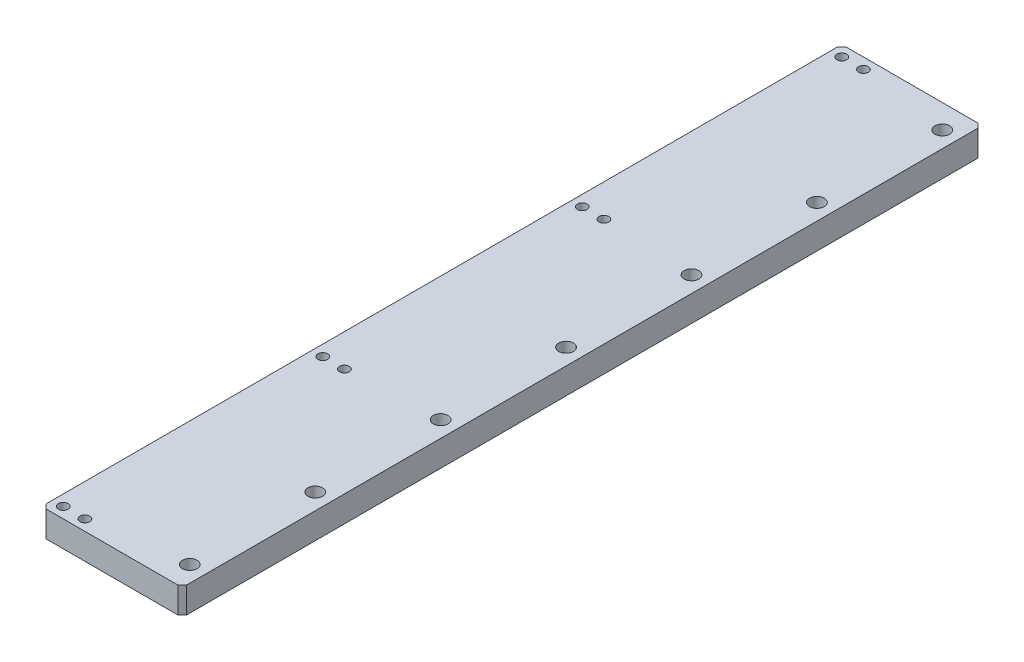
from build123d import *

# Parameters (mm, degrees)
SKETCH_1_W                = 65
SKETCH_1_H                = 370
EXTRUDE_1_DEPTH           = 12
HOLE_WIZARD_M8_1_D        = 6.8
HOLE_WIZARD_1_D           = 4.5
HOLE_WIZARD_1_CBORE_D     = 8
HOLE_WIZARD_1_CBORE_DEPTH = 4.6
CHAMFER_1_SIZE            = 2
PATTERN_LINEAR_1_COUNT    = 2
PATTERN_LINEAR_1_PITCH    = 10


with BuildPart() as part:
    # 草图1 → 凸台-拉伸1 (new body)
    with BuildSketch(Plane(origin=(0, 0, 0), x_dir=(1, 0, 0), z_dir=(0, 1, 0))):
        Rectangle(SKETCH_1_W, SKETCH_1_H)
    extrude(amount=EXTRUDE_1_DEPTH)

    # M8 螺纹孔1 (through all)
    with Locations(Plane(origin=(0, 12, 0), x_dir=(1, 0, 0), z_dir=(0, 1, 0))):
        with Locations((25, -174), (25, -116), (25, -58), (25, 0), (25, 58), (25, 116), (25, 174)):
            Hole(HOLE_WIZARD_M8_1_D / 2)

    # 打孔尺寸(%根据)内六角圆柱头螺钉的类型1 (through all)
    with Locations(Plane(origin=(0, 0, 0), x_dir=(-1, 0, 0), z_dir=(0, -1, 0))):
        with Locations((27.5, -180), (27.5, -60), (27.5, 60), (27.5, 180)):
            hole_wizard_1 = CounterBoreHole(HOLE_WIZARD_1_D / 2, HOLE_WIZARD_1_CBORE_D / 2, HOLE_WIZARD_1_CBORE_DEPTH)

    # 倒角1
    chamfer_1_edges = [part.edges().sort_by_distance(p)[0] for p in [
        (32.5, 6, 185),
        (-32.5, 6, 185),
        (-32.5, 6, -185),
        (32.5, 6, -185),
    ]]
    chamfer(chamfer_1_edges, length=CHAMFER_1_SIZE)

    # 阵列(线性)1: 打孔尺寸(%根据)内六角圆柱头螺钉的类型1 ×2
    with Locations(*[(i * PATTERN_LINEAR_1_PITCH, 0, 0) for i in range(1, PATTERN_LINEAR_1_COUNT)]):
        add(hole_wizard_1, mode=Mode.SUBTRACT)


solid = part.part
